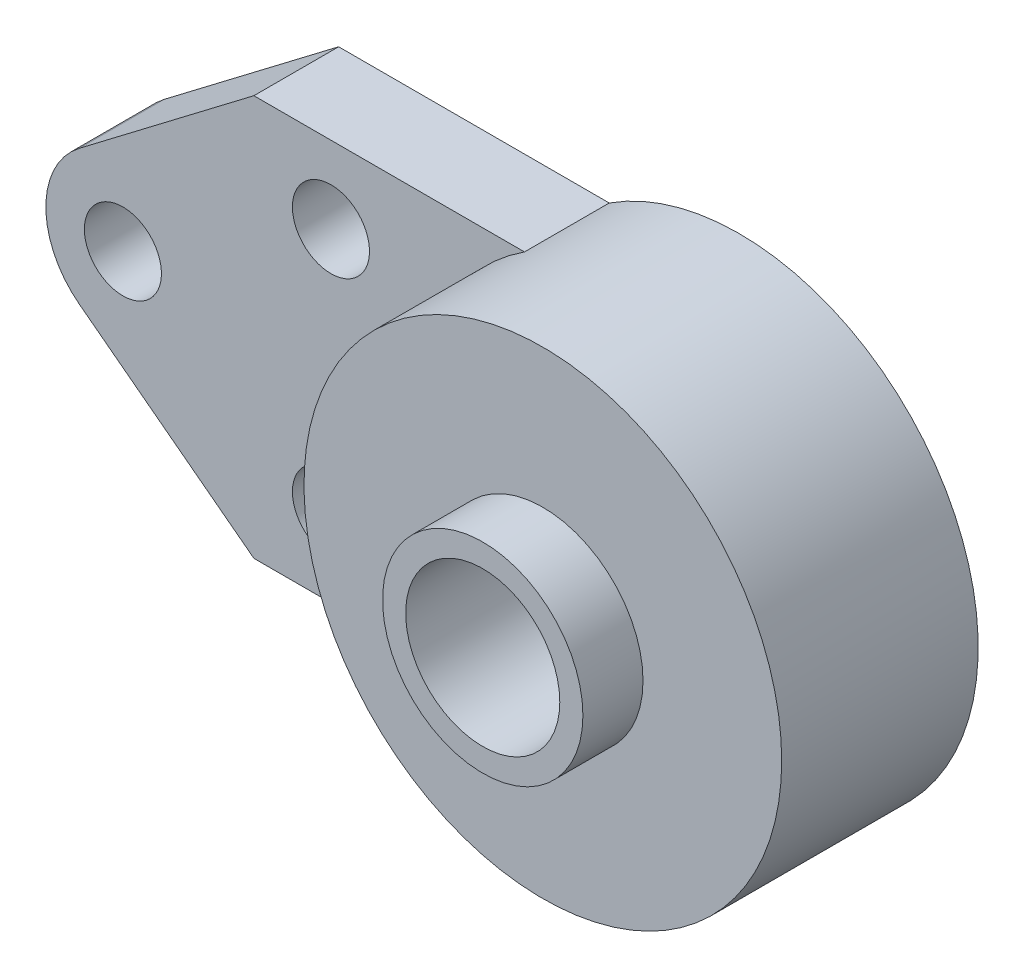
SolidWorks part; units mm, degrees
ref_plane "前视基准面" through (0, 0, 0) normal (0, 0, 1) x (1, 0, 0)
ref_plane "上视基准面" through (0, 0, 0) normal (0, 1, 0) x (1, 0, 0)
ref_plane "右视基准面" through (0, 0, 0) normal (1, 0, 0) x (0, 0, -1)
sketch "草图1" plane through (0, 0, 0) normal (0, 0, 1) x (1, 0, 0)
  circle A0 centre (0, 0) radius 10
  circle A1 centre (0, 0) radius 31
  dimension "D1" = 20
  dimension "D2" = 62
extrude "凸台-拉伸1" add sketch "草图1" along normal blind 25.5
sketch "草图2" plane through (0, 0, 0) normal (0, 0, -1) x (-1, 0, 0)
  line L0 (0, 0) -> (68, 0) construction
  line L1 (16.8819, 26) -> (52, 26)
  line L2 (52, 26) -> (74.6617, 8.7534)
  line L3 (52, -26) -> (74.6617, -8.7534)
  line L4 (16.8819, -26) -> (52, -26)
  line L5 (42, 16) -> (42, 0) construction
  line L6 (42, 0) -> (42, -16) construction
  arc A0 (74.6617, -8.7534) -> (74.6617, 8.7534) centre (68, 0) ccw
  circle A3 centre (0, 0) radius 31 construction
  arc A4 (16.8819, -26) -> (16.8819, 26) centre (0, 0) ccw
  circle A5 centre (69, 0) radius 5
  circle A6 centre (42, 16) radius 5
  circle A7 centre (42, -16) radius 5
  circle A8 centre (0, 0) radius 10 construction
  dimension "D1" = 110
  dimension "D4" = 27
  dimension "D5" = 42
  dimension "D6" = 10
  dimension "D7" = 11
  dimension "D8" = 52
  dimension "D2" = 52
  dimension "D3" = 32
extrude "凸台-拉伸2" add sketch "草图2" against normal blind 11
sketch "草图3" plane through (0, 0, 25.5) normal (0, 0, 1) x (1, 0, 0)
  circle A0 centre (0, 0) radius 13
  circle A1 centre (0, 0) radius 10 construction
  circle A2 centre (0, 0) radius 10
  dimension "D1" = 26
extrude "凸台-拉伸3" add sketch "草图3" along normal blind 7.8
